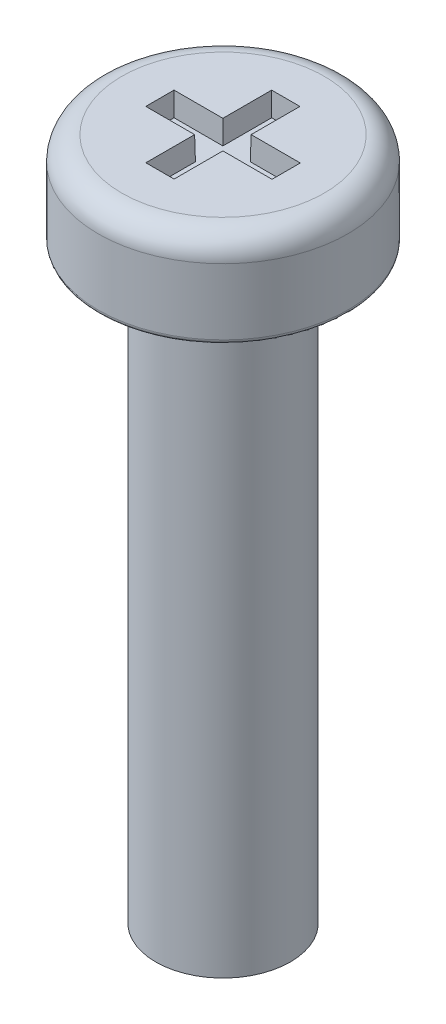
SolidWorks part; units mm, degrees
ref_plane "Front Plane" through (0, 0, 0) normal (0, 0, 1) x (1, 0, 0)
ref_plane "Top Plane" through (0, 0, 0) normal (0, 1, 0) x (1, 0, 0)
ref_plane "Right Plane" through (0, 0, 0) normal (1, 0, 0) x (0, 0, -1)
sketch "Sketch1" plane through (0, 0, 0) normal (0, 1, 0) x (1, 0, 0)
  circle A0 centre (0, 0) radius 2.65
  dimension "D1" = 5.3
extrude "Boss-Extrude1" add sketch "Sketch1" along normal blind 2
sketch "Sketch2" plane through (0, 0, 0) normal (0, -1, 0) x (1, 0, 0)
  circle A0 centre (0, 0) radius 1.43
  dimension "D1" = 2.86
extrude "Boss-Extrude2" add sketch "Sketch2" along normal blind 12.5
fillet "Fillet1" radius 0.5 1 edges at (0, 2, 2.65)
fillet "Fillet2" radius 0.1 1 edges at (0, 0, 2.65)
sketch "Sketch3" plane through (0, 2, 0) normal (0, 1, 0) x (1, 0, 0)
  line L0 (0.2966, 0.3) -> (1.3407, 0.3)
  line L1 (-1.3407, -0.3) -> (-0.3034, -0.3)
  line L2 (-1.3407, -0.3) -> (-1.3407, 0.3)
  line L3 (-1.3407, 0.3) -> (-0.3034, 0.3)
  line L4 (1.3407, -0.3) -> (1.3407, 0.3)
  line L5 (0.2966, 0.3) -> (0.2966, 1.3361)
  line L6 (-1.3472, 0.3015) -> (-1.3407, 0.3) construction
  line L7 (-0.3034, -1.3361) -> (0.2966, -1.3361)
  line L8 (-0.3034, -1.3361) -> (-0.3034, -0.3)
  line L9 (-0.3034, 1.3361) -> (0.2966, 1.3361)
  line L10 (0.2966, -1.3361) -> (0.2966, -0.3)
  line L11 (-0.0036, -0.0008) -> (-0.0033, 0.0007) construction
  line L12 (-0.0033, 0.0007) -> (-0.003, -0.0007) construction
  line L13 (-0.3034, 0.3) -> (-0.3034, 1.3361)
  line L15 (0.2966, -0.3) -> (1.3407, -0.3)
  line L17 (-0.0036, -0.0008) -> (0, 0) construction
  line L18 (-0.0033, 0.0007) -> (0, 0) construction
  point P0 (0, 0)
  point P6 (-0.0033, 0.0007)
  dimension "D1" = 0.6
  dimension "D2" = 0.6
extrude "Cut-Extrude1" cut sketch "Sketch3" against normal blind 0.5 draft 1
sketch "Sketch4" plane through (0, -12.5, 0) normal (0, -1, 0) x (1, 0, 0)
  circle A1 centre (0, 0) radius 1.43
  circle A2 centre (0, 0) radius 1.43
  dimension "D1" = 0
curve "Helix/Spiral1" pitch 0.3 height 5 turns 16.6667
